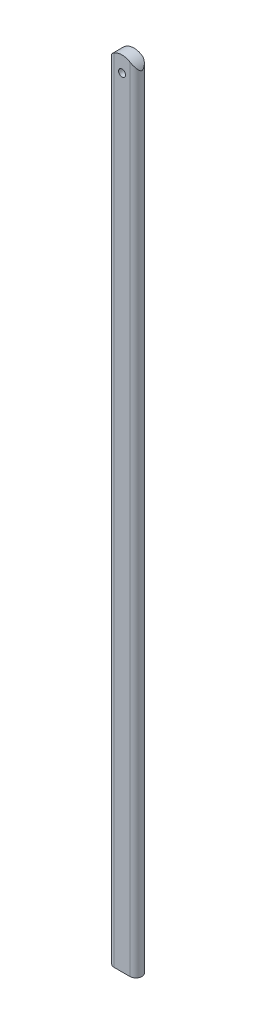
from build123d import *

# Parameters (mm, degrees)
BOSS_EXTRUDE1_DEPTH = 400
CUT_EXTRUDE1_DEPTH  = 401.196201881
SKETCH3_R           = 1.75
CUT_EXTRUDE2_DEPTH  = 401.196201985


with BuildPart() as part:
    # Sketch1 → Boss-Extrude1 (new body)
    with BuildSketch(Plane(origin=(0, 0, 0), x_dir=(1, 0, 0), z_dir=(0, 1, 0))):
        with BuildLine():
            Line((0, 3), (8, 3))
            ThreePointArc((8, 3), (11, 0), (8, -3))
            Line((8, -3), (0, -3))
            ThreePointArc((0, -3), (-3, 0), (0, 3))
        make_face()
    extrude(amount=-BOSS_EXTRUDE1_DEPTH)

    # Sketch2 → Cut-Extrude1 (cut, through all)
    with BuildSketch(Plane(origin=(0, 0, -3), x_dir=(-1, 0, 0), z_dir=(0, 0, -1))):
        with BuildLine():
            Line((9.595782006, 3.055219164), (9.595782006, -10.123279697))
            Line((9.595782006, -10.123279697), (3.026265269, -10.123279697))
            ThreePointArc((3.026265269, -10.123279697), (-4, 0), (-11.026265269, -10.123279697))
            Line((-11.026265269, -10.123279697), (-18.139014199, -10.123279697))
            Line((-18.139014199, -10.123279697), (-18.139014199, 3.055219164))
            Line((-18.139014199, 3.055219164), (9.595782006, 3.055219164))
        make_face()
    extrude(amount=-CUT_EXTRUDE1_DEPTH, mode=Mode.SUBTRACT)

    # Sketch3 → Cut-Extrude2 (cut, through all)
    with BuildSketch(Plane.XY.offset(3)):
        with Locations((4, -7.883965637)):
            Circle(SKETCH3_R)
    extrude(amount=-CUT_EXTRUDE2_DEPTH, mode=Mode.SUBTRACT)


solid = part.part
